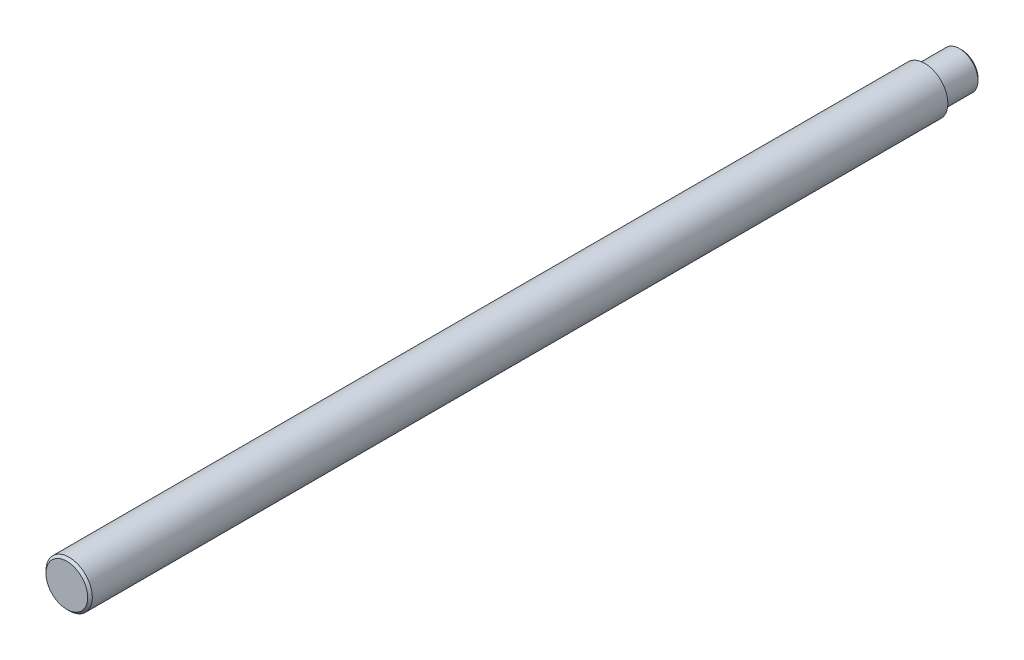
from build123d import *

# Parameters (mm, degrees)
SKETCH_1_R      = 5
EXTRUDE_1_DEPTH = 185
SKETCH_2_R      = 4
EXTRUDE_2_DEPTH = 8
CHAMFER_1_SIZE  = 0.5


with BuildPart() as part:
    # 草图1 → 凸台-拉伸1 (new body)
    with BuildSketch(Plane.XY):
        Circle(SKETCH_1_R)
    extrude(amount=EXTRUDE_1_DEPTH)

    # 草图2 → 凸台-拉伸2 (add)
    with BuildSketch(Plane(origin=(0, 0, 0), x_dir=(-1, 0, 0), z_dir=(0, 0, -1))):
        with Locations(Location((0, 0, 0), (0, 0, 180))):
            Circle(SKETCH_2_R)
    extrude(amount=EXTRUDE_2_DEPTH)

    # 倒角1
    chamfer_1_edges = [part.edges().sort_by_distance(p)[0] for p in [
        (-5, 0, 185),
        (-4, 0, -8),
    ]]
    chamfer(chamfer_1_edges, length=CHAMFER_1_SIZE)


solid = part.part
